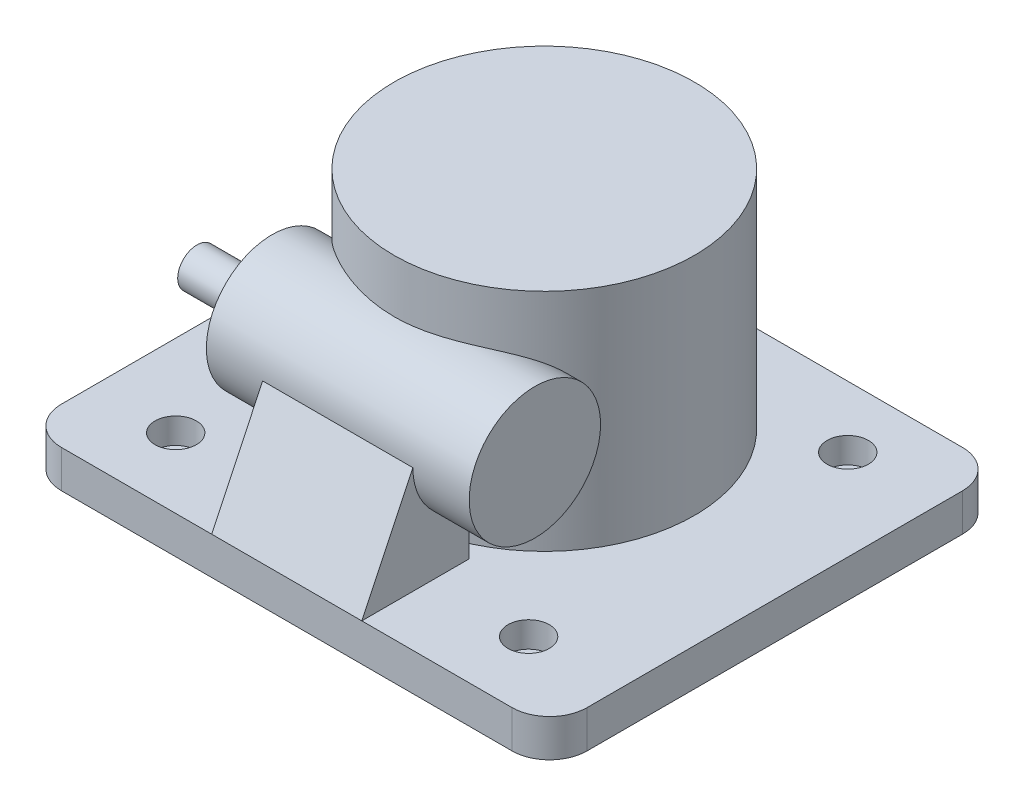
from build123d import *

# Parameters (mm, degrees)
SKETCH1_R                                   = 40
BOSS_EXTRUDE1_DEPTH                         = 60
SKETCH2_W                                   = 140
SKETCH2_H                                   = 120
BOSS_EXTRUDE2_DEPTH                         = 10
SKETCH3_R                                   = 17.5
BOSS_EXTRUDE3_DEPTH                         = 35
BOSS_EXTRUDE6_DEPTH                         = 20
FILLET1_R                                   = 10
HOLE_SIZE_PER_SOCKET_HEAD_CAP_SCREW_2_COUNT = 2
HOLE_SIZE_PER_SOCKET_HEAD_CAP_SCREW_2_PITCH = 85
HOLE_SIZE_PER_SOCKET_HEAD_CAP_SCREW_3_COUNT = 2
HOLE_SIZE_PER_SOCKET_HEAD_CAP_SCREW_3_PITCH = 126.732000694
HOLE_SIZE_PER_SOCKET_HEAD_CAP_SCREW_4_COUNT = 2
HOLE_SIZE_PER_SOCKET_HEAD_CAP_SCREW_4_PITCH = 94
SKETCH10_R                                  = 5.135329367
BOSS_EXTRUDE7_DEPTH                         = 20


with BuildPart() as part:
    # Sketch1 → Boss-Extrude1 (new body)
    with BuildSketch(Plane(origin=(0, 0, 0), x_dir=(1, 0, 0), z_dir=(0, 1, 0))):
        with Locations(Location((0, 0, 0), (0, 0, 270))):
            Circle(SKETCH1_R)
    extrude(amount=BOSS_EXTRUDE1_DEPTH)

    # Sketch2 → Boss-Extrude2 (add)
    with BuildSketch(Plane.XZ):
        with Locations((0, 8.595087693)):
            Rectangle(SKETCH2_W, SKETCH2_H)
    extrude(amount=BOSS_EXTRUDE2_DEPTH)

    # Sketch3 → Boss-Extrude3 (add, symmetric)
    with BuildSketch(Plane(origin=(0, 0, 0), x_dir=(0, 0, -1), z_dir=(1, 0, 0))):
        with Locations((-37.50111495, 28.542378204)):
            Circle(SKETCH3_R)
    extrude(amount=BOSS_EXTRUDE3_DEPTH, both=True)

    # Fillet1
    fillet1_edges = [part.edges().sort_by_distance(p)[0] for p in [
        (70, -5, -51.404912307),
        (70, -5, 68.595087693),
        (-70, -5, 68.595087693),
        (-70, -5, -51.404912307),
    ]]
    fillet(fillet1_edges, radius=FILLET1_R)

    # Sketch9 → Hole size per socket head cap screw type1 (revolve, cut)
    with BuildSketch(Plane(origin=(-48.166410727, 0, 50), x_dir=(0, 0, 1), z_dir=(1, 0, 0))):
        Polygon((0, 0), (0, 10), (3.3, 10), (3.3, 6.8), (5.5, 6.8), (5.5, 0), align=None)
    hole_size_per_socket_head_cap_screw_type = revolve(axis=Axis((-48.166410727, 6.35, 50), (0, -1, 0)), mode=Mode.SUBTRACT)

    # Hole size per socket head cap screw  2: Hole size per socket head cap screw type1 ×2
    with Locations(*[(0, 0, -i * HOLE_SIZE_PER_SOCKET_HEAD_CAP_SCREW_2_PITCH) for i in range(1, HOLE_SIZE_PER_SOCKET_HEAD_CAP_SCREW_2_COUNT)]):
        add(hole_size_per_socket_head_cap_screw_type, mode=Mode.SUBTRACT)

    # Hole size per socket head cap screw  3: Hole size per socket head cap screw type1 ×2
    with Locations(*[Vector(0.741722686337812, 0, -0.6707066844544043) * (i * HOLE_SIZE_PER_SOCKET_HEAD_CAP_SCREW_3_PITCH) for i in range(1, HOLE_SIZE_PER_SOCKET_HEAD_CAP_SCREW_3_COUNT)]):
        add(hole_size_per_socket_head_cap_screw_type, mode=Mode.SUBTRACT)

    # Hole size per socket head cap screw  4: Hole size per socket head cap screw type1 ×2
    with Locations(*[(i * HOLE_SIZE_PER_SOCKET_HEAD_CAP_SCREW_4_PITCH, 0, 0) for i in range(1, HOLE_SIZE_PER_SOCKET_HEAD_CAP_SCREW_4_COUNT)]):
        add(hole_size_per_socket_head_cap_screw_type, mode=Mode.SUBTRACT)

    # Sketch10 → Boss-Extrude7 (add)
    with BuildSketch(Plane.ZY.offset(35)):
        with Locations(Location((37.50111495, 28.542378204, 0), (0, 0, 180))):
            Circle(SKETCH10_R)
    extrude(amount=BOSS_EXTRUDE7_DEPTH)


with BuildPart() as body_2:
    # Sketch4 → Boss-Extrude6 (new, symmetric)
    with BuildSketch(Plane(origin=(0, 0, 0), x_dir=(0, 0, -1), z_dir=(1, 0, 0))):
        with BuildLine():
            Line((-55.00111495, 28.542378204), (-68.595087693, 0))
            Line((-68.595087693, 0), (-40, 0))
            Line((-40, 0), (-40, 11.221709236))
            ThreePointArc((-40, 11.221709236), (-50.729502765, 17.085513196), (-55.00111495, 28.542378204))
        make_face()
    extrude(amount=BOSS_EXTRUDE6_DEPTH, both=True)


solid = Compound([part.part, body_2.part])
